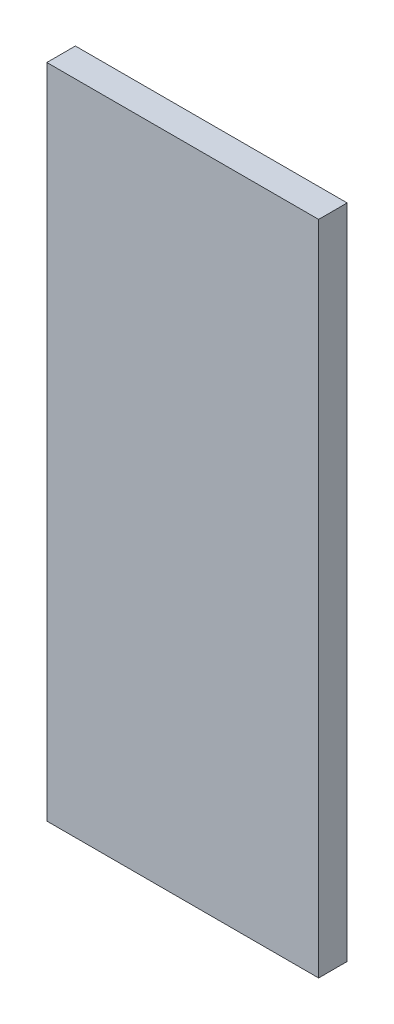
SolidWorks part; units mm, degrees
material "普通碳钢"
ref_plane "Front Plane" through (0, 0, 0) normal (0, 0, 1) x (1, 0, 0)
ref_plane "Top Plane" through (0, 0, 0) normal (0, 1, 0) x (1, 0, 0)
ref_plane "Right Plane" through (0, 0, 0) normal (1, 0, 0) x (0, 0, -1)
sketch "Sketch1" plane through (0, 0, 0) normal (0, 0, 1) x (1, 0, 0)
  line L1 (-38.1, 92.1) -> (38.1, 92.1)
  line L2 (-38.1, 92.1) -> (-38.1, -92.1)
  line L3 (-38.1, -92.1) -> (38.1, -92.1)
  line L4 (38.1, 92.1) -> (38.1, -92.1)
  dimension "D1" = 184.2
  dimension "D2" = 92.1
  dimension "D3" = 76.2
  dimension "D4" = 38.1
extrude "Boss-Extrude1" add sketch "Sketch1" along normal mid plane 8
